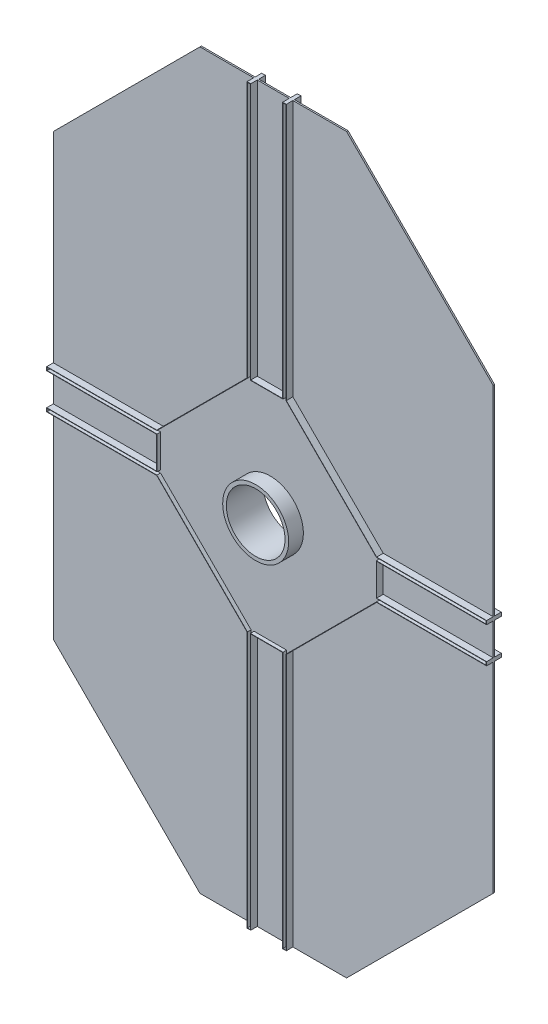
from build123d import *

# Parameters (mm, degrees)
SKETCH1_R                = 45
SKETCH1_R_2              = 40
BOSS_EXTRUDE1_DEPTH      = 50
BOSS_EXTRUDE2_START      = 10
SKETCH4_R                = 45
BOSS_EXTRUDE2_DEPTH      = 10
BOSS_EXTRUDE3_START      = -4
SKETCH6_W                = 200
SKETCH6_H                = 600
SKETCH6_H_2              = 200
SKETCH6_R                = 40
BOSS_EXTRUDE3_DEPTH      = 2
SKETCH7_W                = 150
SKETCH7_H                = 5
SKETCH7_W_2              = 5
SKETCH7_H_2              = 350
BOSS_EXTRUDE4_DEPTH      = 10
EXTRUDE_THIN2_DEPTH      = 5
EXTRUDE_THIN2_DEPTH_BACK = 15


with BuildPart() as part:
    # Sketch1 → Boss-Extrude1 (new body)
    with BuildSketch(Plane.XY):
        with Locations((-599.884196758, -90)):
            Circle(SKETCH1_R)
        with Locations((-599.884196758, -90)):
            Circle(SKETCH1_R_2, mode=Mode.SUBTRACT)
    extrude(amount=BOSS_EXTRUDE1_DEPTH)

    # Sketch4 → Boss-Extrude2 (add)
    with BuildSketch(Plane(origin=(0, 0, 30), x_dir=(-1, 0, 0), z_dir=(0, 0, -1)).offset(BOSS_EXTRUDE2_START)):
        Polygon((626.660892055, -240), (749.884196758, -116.776695297), (749.884196758, -63.223304703), (626.660892055, 60), (573.107501461, 60), (449.884196758, -63.223304703), (449.884196758, -116.776695297), (573.107501461, -240), align=None)
        with Locations(Location((599.884196758, -90, 0), (0, 0, 180))):
            Circle(SKETCH4_R, mode=Mode.SUBTRACT)
    extrude(amount=-BOSS_EXTRUDE2_DEPTH)

    # Sketch6 → Boss-Extrude3 (add)
    # profile 1 of 9: a face of its own
    with BuildSketch(Plane(origin=(0, 0, 20), x_dir=(-1, 0, 0), z_dir=(0, 0, -1)).offset(BOSS_EXTRUDE3_START)):
        with Locations((799.884196758, -90)):
            Rectangle(SKETCH6_W, SKETCH6_H)
    # profile 2 of 9: a face of its own
    with BuildSketch(Plane(origin=(0, 0, 20), x_dir=(-1, 0, 0), z_dir=(0, 0, -1)).offset(BOSS_EXTRUDE3_START)):
        Polygon((699.884196758, -590), (899.884196758, -390), (699.884196758, -390), align=None)
    # profile 3 of 9: a face of its own
    with BuildSketch(Plane(origin=(0, 0, 20), x_dir=(-1, 0, 0), z_dir=(0, 0, -1)).offset(BOSS_EXTRUDE3_START)):
        with Locations((599.884196758, -490)):
            Rectangle(SKETCH6_W, SKETCH6_H_2)
    # profile 4 of 9: a face of its own
    with BuildSketch(Plane(origin=(0, 0, 20), x_dir=(-1, 0, 0), z_dir=(0, 0, -1)).offset(BOSS_EXTRUDE3_START)):
        Polygon((699.884196758, 210), (899.884196758, 210), (699.884196758, 410), align=None)
    # profile 5 of 9: a face of its own
    with BuildSketch(Plane(origin=(0, 0, 20), x_dir=(-1, 0, 0), z_dir=(0, 0, -1)).offset(BOSS_EXTRUDE3_START)):
        with Locations((599.884196758, -90)):
            Rectangle(SKETCH6_W, SKETCH6_H)
        with Locations(Location((599.884196758, -90, 0), (0, 0, 180))):
            Circle(SKETCH6_R, mode=Mode.SUBTRACT)
    # profile 6 of 9: a face of its own
    with BuildSketch(Plane(origin=(0, 0, 20), x_dir=(-1, 0, 0), z_dir=(0, 0, -1)).offset(BOSS_EXTRUDE3_START)):
        Polygon((299.884196758, -390), (499.884196758, -590), (499.884196758, -390), align=None)
    # profile 7 of 9: a face of its own
    with BuildSketch(Plane(origin=(0, 0, 20), x_dir=(-1, 0, 0), z_dir=(0, 0, -1)).offset(BOSS_EXTRUDE3_START)):
        with Locations((599.884196758, 310)):
            Rectangle(SKETCH6_W, SKETCH6_H_2)
    # profile 8 of 9: a face of its own
    with BuildSketch(Plane(origin=(0, 0, 20), x_dir=(-1, 0, 0), z_dir=(0, 0, -1)).offset(BOSS_EXTRUDE3_START)):
        with Locations((399.884196758, -90)):
            Rectangle(SKETCH6_W, SKETCH6_H)
    # profile 9 of 9: a face of its own
    with BuildSketch(Plane(origin=(0, 0, 20), x_dir=(-1, 0, 0), z_dir=(0, 0, -1)).offset(BOSS_EXTRUDE3_START)):
        Polygon((299.884196758, 210), (499.884196758, 210), (499.884196758, 410), align=None)
    extrude(amount=-BOSS_EXTRUDE3_DEPTH)

    # Sketch7 → Boss-Extrude4 (add)
    with BuildSketch(Plane(origin=(0, 0, 20), x_dir=(-1, 0, 0), z_dir=(0, 0, -1))):
        with Locations((824.884196758, -65.723304703)):
            Rectangle(SKETCH7_W, SKETCH7_H)
        with Locations((824.884196758, -114.276695297)):
            Rectangle(SKETCH7_W, SKETCH7_H)
        with Locations((374.884196758, -114.276695297)):
            Rectangle(SKETCH7_W, SKETCH7_H)
        with Locations((374.884196758, -65.723304703)):
            Rectangle(SKETCH7_W, SKETCH7_H)
        with Locations((624.160892055, -415)):
            Rectangle(SKETCH7_W_2, SKETCH7_H_2)
        with Locations((575.607501461, -415)):
            Rectangle(SKETCH7_W_2, SKETCH7_H_2)
        with Locations((575.607501461, 235)):
            Rectangle(SKETCH7_W_2, SKETCH7_H_2)
        with Locations((624.160892055, 235)):
            Rectangle(SKETCH7_W_2, SKETCH7_H_2)
    extrude(amount=-BOSS_EXTRUDE4_DEPTH)

    # Sketch8 → Extrude-Thin2 (add, two sides: drawn at the far end of the back side and taken through both)
    with BuildSketch(Plane(origin=(0, 0, 20), x_dir=(-1, 0, 0), z_dir=(0, 0, -1)).offset(-EXTRUDE_THIN2_DEPTH_BACK)):
        Polygon((749.884196758, -63.223304703), (626.660892055, 60), (626.660892055, 410), (621.660892055, 410), (621.660892055, 60), (578.107501461, 60), (578.107501461, 410), (573.107501461, 410), (573.107501461, 60), (449.884196758, -63.223304703), (299.884196758, -63.223304703), (299.884196758, -68.223304703), (449.884196758, -68.223304703), (449.884196758, -111.776695297), (299.884196758, -111.776695297), (299.884196758, -116.776695297), (449.884196758, -116.776695297), (573.107501461, -240), (573.107501461, -590), (578.107501461, -590), (578.107501461, -240), (621.660892055, -240), (621.660892055, -590), (626.660892055, -590), (626.660892055, -240), (749.884196758, -116.776695297), (899.884196758, -116.776695297), (899.884196758, -111.776695297), (749.884196758, -111.776695297), (749.884196758, -68.223304703), (899.884196758, -68.223304703), (899.884196758, -63.223304703), align=None)
        Polygon((749.677089977, -63.723304703), (626.160892055, 59.792893219), (626.160892055, 409.5), (622.160892055, 409.5), (622.160892055, 59.5), (577.607501461, 59.5), (577.607501461, 409.5), (573.607501461, 409.5), (573.607501461, 59.792893219), (450.091303539, -63.723304703), (300.384196758, -63.723304703), (300.384196758, -67.723304703), (450.384196758, -67.723304703), (450.384196758, -112.276695297), (300.384196758, -112.276695297), (300.384196758, -116.276695297), (450.091303539, -116.276695297), (573.607501461, -239.792893219), (573.607501461, -589.5), (577.607501461, -589.5), (577.607501461, -239.5), (622.160892055, -239.5), (622.160892055, -589.5), (626.160892055, -589.5), (626.160892055, -239.792893219), (749.677089977, -116.276695297), (899.384196758, -116.276695297), (899.384196758, -112.276695297), (749.384196758, -112.276695297), (749.384196758, -67.723304703), (899.384196758, -67.723304703), (899.384196758, -63.723304703), align=None, mode=Mode.SUBTRACT)
    extrude(amount=EXTRUDE_THIN2_DEPTH + EXTRUDE_THIN2_DEPTH_BACK)


solid = part.part
